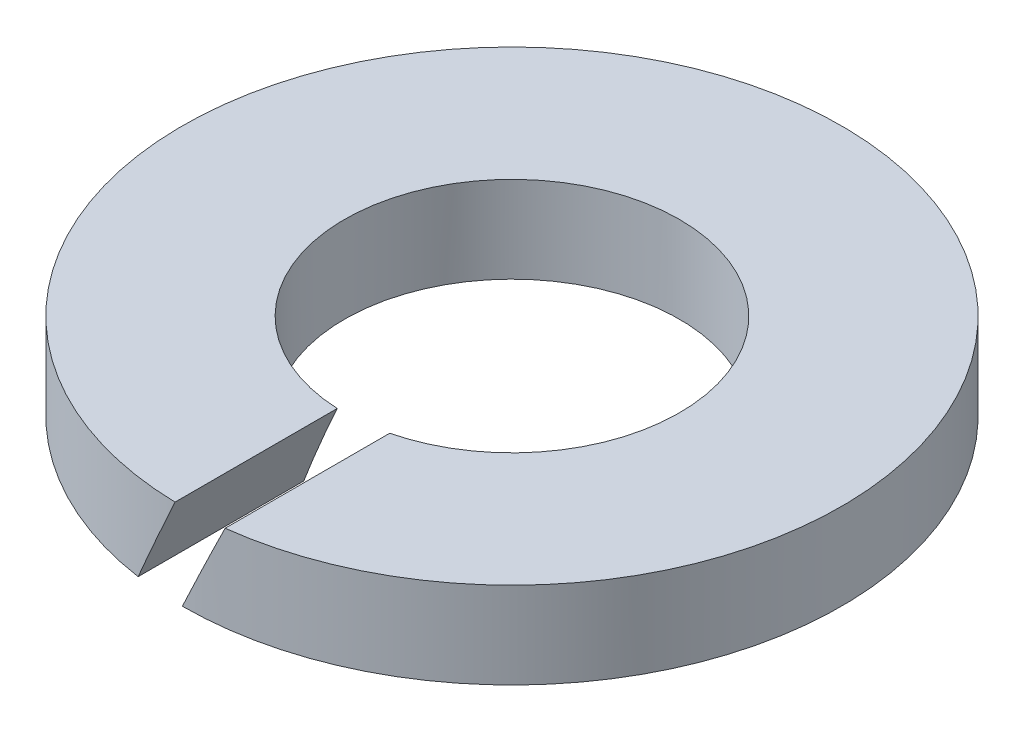
from build123d import *

# Parameters (mm, degrees)
SKETCH_1_R          = 3.05
SKETCH_1_R_2        = 1.55
EXTRUDE_1_DEPTH     = 0.8
CUT_EXTRUDE_1_DEPTH = 5.386912354


with BuildPart() as part:
    # 草图1 → 凸台-拉伸1 (new body)
    with BuildSketch(Plane(origin=(0, 0, 0), x_dir=(1, 0, 0), z_dir=(0, 1, 0))):
        with Locations(Location((0, 0, 0), (0, 0, 270))):
            Circle(SKETCH_1_R)
        with Locations(Location((0, 0, 0), (0, 0, 270))):
            Circle(SKETCH_1_R_2, mode=Mode.SUBTRACT)
    extrude(amount=EXTRUDE_1_DEPTH)

    # 草图2 → 切除-拉伸1 (cut, through all)
    with BuildSketch(Plane.XY):
        Polygon((0, 0), (0.373046127, 0.8), (-0.068305041, 0.8), (-0.441351168, 0), align=None)
    extrude(amount=CUT_EXTRUDE_1_DEPTH, mode=Mode.SUBTRACT)


solid = part.part
